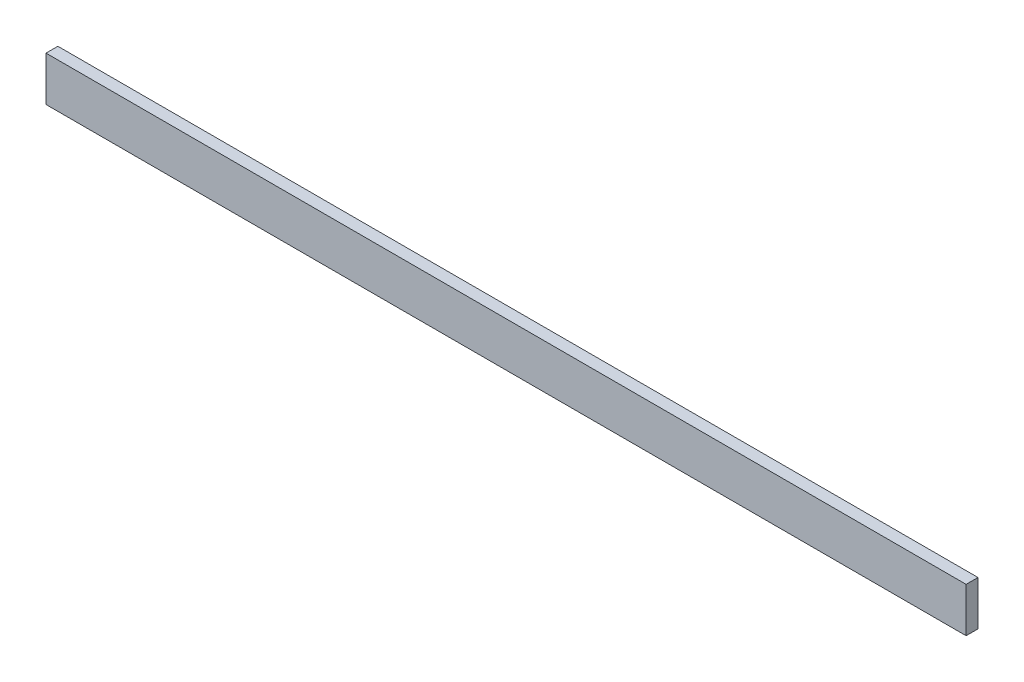
SolidWorks part; units mm, degrees
ref_plane "Front Plane" through (0, 0, 0) normal (0, 0, 1) x (1, 0, 0)
ref_plane "Top Plane" through (0, 0, 0) normal (0, 1, 0) x (1, 0, 0)
ref_plane "Right Plane" through (0, 0, 0) normal (1, 0, 0) x (0, 0, -1)
sketch "Sketch1" plane through (0, 0, 0) normal (0, 0, 1) x (1, 0, 0)
  line L1 (0, 0) -> (620, 0)
  line L2 (0, 0) -> (0, 30)
  line L3 (0, 30) -> (620, 30)
  line L4 (620, 0) -> (620, 30)
  dimension "D1" = 620
  dimension "D2" = 30
extrude "Boss-Extrude1" add sketch "Sketch1" along normal blind 8
